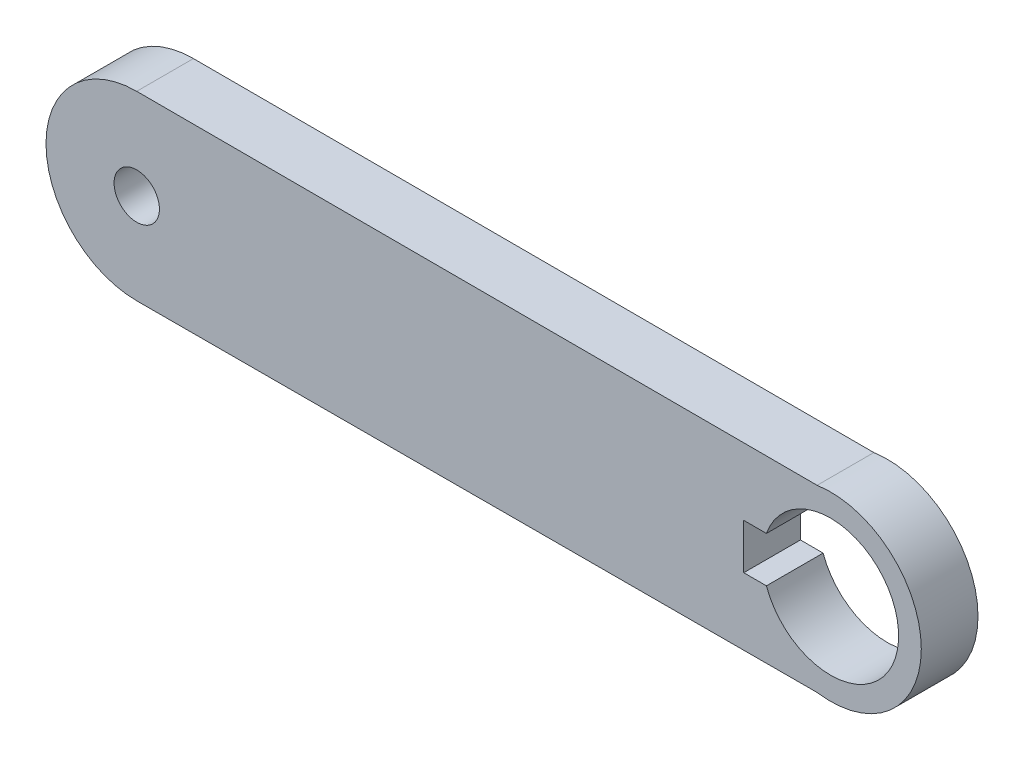
from build123d import *

# Parameters (mm, degrees)
SKETCH_1_R      = 2
EXTRUDE_1_DEPTH = 5


with BuildPart() as part:
    # 草图1 → 凸台-拉伸1 (new body)
    with BuildSketch(Plane.XY):
        with BuildLine():
            Line((-53.730833149, 7.731344519), (6.269166851, 7.643135881))
            ThreePointArc((6.269166851, 7.643135881), (15.453885145, -0.268655481), (6.269166851, -8.180446844))
            Line((6.269166851, -8.180446844), (-53.730833149, -8.268655481))
            ThreePointArc((-53.730833149, -8.268655481), (-61.730833149, -0.268655481), (-53.730833149, 7.731344519))
        make_face()
        with Locations((-53.730833149, -0.268655481)):
            Circle(SKETCH_1_R, mode=Mode.SUBTRACT)
        with BuildLine():
            Line((-0.202969104, 1.731344519), (-0.202969104, -2.268655481))
            Line((-0.202969104, -2.268655481), (1.797030896, -2.268655481))
            ThreePointArc((1.797030896, -2.268655481), (13.453885145, -0.268655481), (1.797030896, 1.731344519))
            Line((1.797030896, 1.731344519), (-0.202969104, 1.731344519))
        make_face(mode=Mode.SUBTRACT)
    extrude(amount=EXTRUDE_1_DEPTH)


solid = part.part
